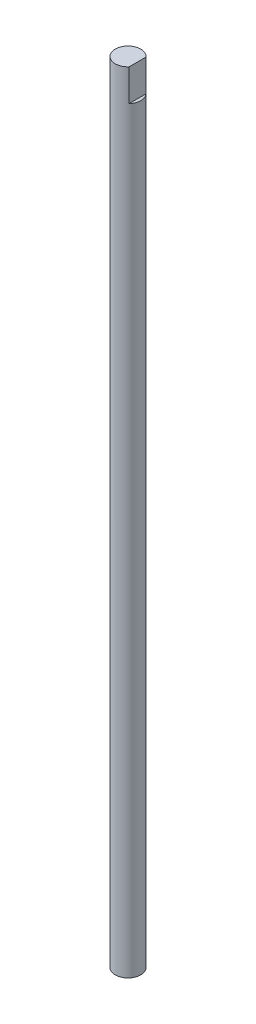
from build123d import *

# Parameters (mm, degrees)
SKETCH1_R               = 8
BOSS_EXTRUDE1_DEPTH     = 495
CUT_EXTRUDE1_DEPTH      = 496.129276048
CUT_EXTRUDE1_DEPTH_BACK = 496.129276048
SKETCH2_W               = 2
SKETCH2_H               = 20


with BuildPart() as part:
    # Sketch1 → Boss-Extrude1 (new body)
    with BuildSketch(Plane(origin=(0, 0, 0), x_dir=(1, 0, 0), z_dir=(0, 1, 0))):
        with Locations(Location((0, 0, 0), (0, 0, 270))):
            Circle(SKETCH1_R)
    extrude(amount=BOSS_EXTRUDE1_DEPTH)

    # Sketch2 → Cut-Extrude1 (cut, two sides: drawn at the far end of the back side and taken through both)
    with BuildSketch(Plane.XY.offset(-CUT_EXTRUDE1_DEPTH_BACK)):
        with Locations((7, 485)):
            Rectangle(SKETCH2_W, SKETCH2_H)
    extrude(amount=CUT_EXTRUDE1_DEPTH + CUT_EXTRUDE1_DEPTH_BACK, mode=Mode.SUBTRACT)


solid = part.part
